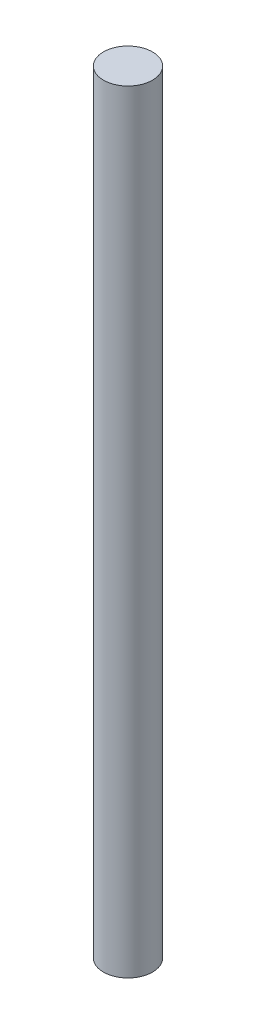
SolidWorks part; units mm, degrees
ref_plane "Front Plane" through (0, 0, 0) normal (0, 0, 1) x (1, 0, 0)
ref_plane "Top Plane" through (0, 0, 0) normal (0, 1, 0) x (1, 0, 0)
ref_plane "Right Plane" through (0, 0, 0) normal (1, 0, 0) x (0, 0, -1)
sketch "Sketch1" plane through (0, 0, 0) normal (0, 1, 0) x (1, 0, 0)
  circle A0 centre (0, 0) radius 3.175
  dimension "D1" = 6.35
extrude "Boss-Extrude1" add sketch "Sketch1" along normal blind 100
